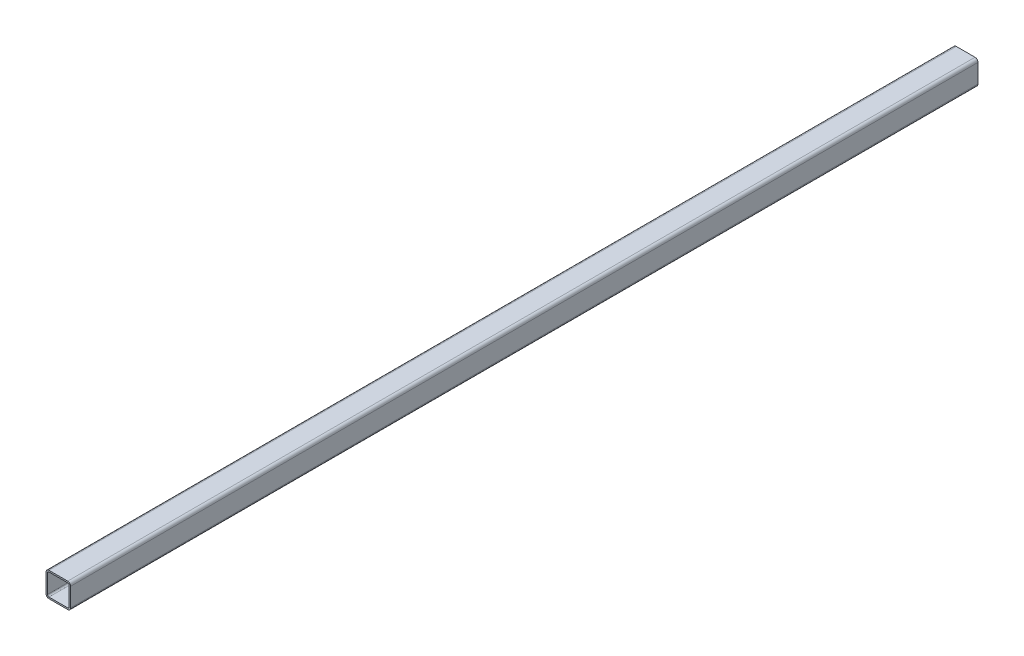
SolidWorks part; units mm, degrees
material "Q235B"
ref_plane "前视基准面" through (0, 0, 0) normal (0, 0, 1) x (1, 0, 0)
ref_plane "上视基准面" through (0, 0, 0) normal (0, 1, 0) x (1, 0, 0)
ref_plane "右视基准面" through (0, 0, 0) normal (1, 0, 0) x (0, 0, -1)
other "Configuration Table"
sketch "草图1" plane through (0, 0, 0) normal (1, 0, 0) x (0, 0, -1)
  line L0 (-920, 0) -> (920, 0)
other "Gb／6728-1986方形空心型钢 050 X 50 X 3(1)"
ref_plane "基准面1" through (0, 0, 920) normal (0, 0, -1) x (0, 1, 0)
sketch "Sketch1" plane through (0, 0, 920) normal (0, 0, -1) x (0, 1, 0)
  line L0 (-19, -22) -> (19, -22)
  line L1 (-22, -19) -> (-22, 19)
  line L2 (19, 22) -> (-19, 22)
  line L3 (22, 19) -> (22, -19)
  line L4 (-19, -25) -> (19, -25)
  line L5 (-25, -19) -> (-25, 19)
  line L6 (19, 25) -> (-19, 25)
  line L7 (25, 19) -> (25, -19)
  arc A0 (25, 19) -> (19, 25) centre (19, 19) ccw
  arc A1 (19, -25) -> (25, -19) centre (19, -19) ccw
  arc A2 (-25, -19) -> (-19, -25) centre (-19, -19) ccw
  arc A3 (-19, 25) -> (-25, 19) centre (-19, 19) ccw
  arc A4 (-19, 22) -> (-22, 19) centre (-19, 19) ccw
  arc A5 (22, 19) -> (19, 22) centre (19, 19) ccw
  arc A6 (19, -22) -> (22, -19) centre (19, -19) ccw
  arc A7 (-22, -19) -> (-19, -22) centre (-19, -19) ccw
  point P0 (-25, 0)
  point P1 (25, 0)
  point P2 (0, 25)
  point P3 (0, -25)
  point P4 (0, 0)
  point P5 (-25, -25)
  point P6 (25, -25)
  point P7 (25, 25)
  point P8 (-25, 25)
  point P33 (0, 0)
  dimension "D1" = 6
  dimension "Thickness" = 3
  dimension "V_leg" = 50
equation "\"D2@草图1\"=\"D1@草图1\"/2"
